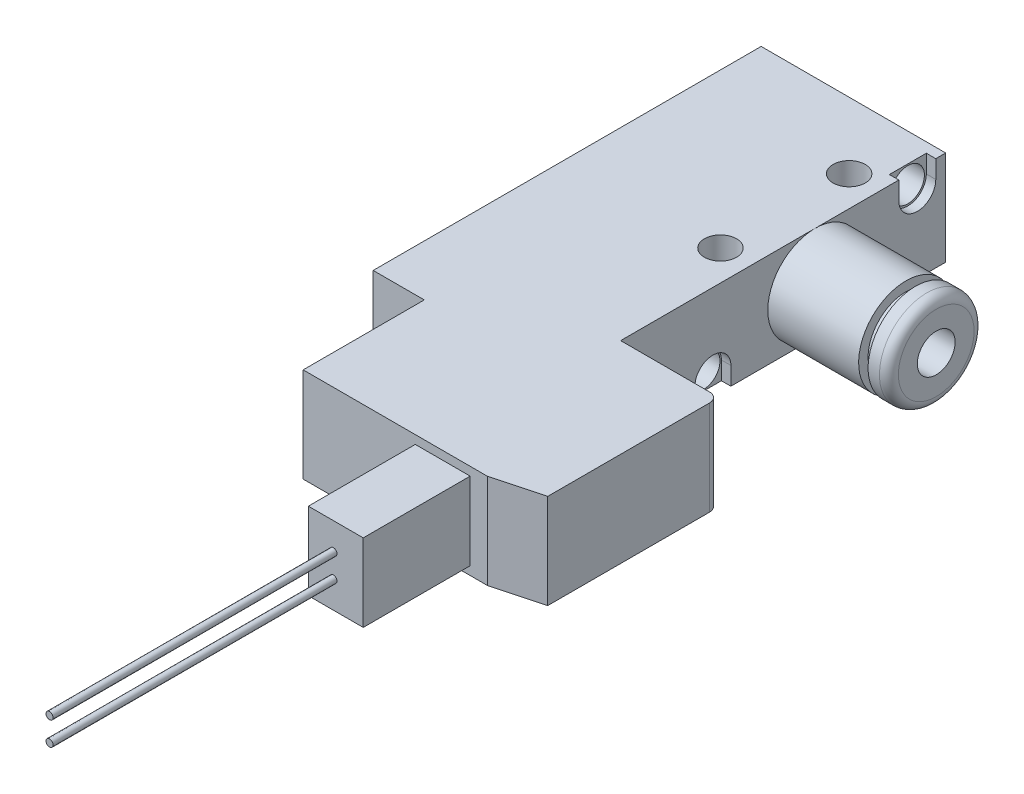
SolidWorks part; units mm, degrees
ref_plane "Front Plane" through (0, 0, 0) normal (0, 0, 1) x (1, 0, 0)
ref_plane "Top Plane" through (0, 0, 0) normal (0, 1, 0) x (1, 0, 0)
ref_plane "Right Plane" through (0, 0, 0) normal (1, 0, 0) x (0, 0, -1)
sketch "Sketch1" plane through (0, 0, 0) normal (1, 0, 0) x (0, 0, -1)
  line L1 (-26.9, 5) -> (26.9, 5)
  line L2 (-26.9, 5) -> (-26.9, -5)
  line L3 (-26.9, -5) -> (26.9, -5)
  line L4 (26.9, 5) -> (26.9, -5)
  line L5 (-26.9, 5) -> (26.9, -5) construction
  line L6 (-26.9, -5) -> (26.9, 5) construction
  point P0 (0, 0)
  dimension "D1" = 53.8
  dimension "D2" = 10
extrude "Boss-Extrude1" add sketch "Sketch1" along normal blind 29.9
sketch "Sketch2" plane through (0, -5, 0) normal (0, -1, 0) x (1, 0, 0)
  line L0 (29.9, -26.9) -> (0, -26.9) construction
  line L1 (0, 26.9) -> (0, -26.9) construction
  circle A0 centre (16.3, -19.9) radius 1.7
  circle A1 centre (16.3, -6.3) radius 1.7
  dimension "D1" = 13.6
  dimension "D3" = 3.4
  dimension "D4" = 3.4
  dimension "D2" = 7
  dimension "D5" = 16.3
extrude "Cut-Extrude1" cut sketch "Sketch2" against normal blind 29.9
sketch "Sketch3" plane through (0, 0, 26.9) normal (0, 0, 1) x (1, 0, 0)
  line L1 (0, 5) -> (0, -5) construction
  line L2 (17.25, 4.1) -> (23.05, 4.1)
  line L3 (17.25, 4.1) -> (17.25, -4.1)
  line L4 (17.25, -4.1) -> (23.05, -4.1)
  line L5 (23.05, 4.1) -> (23.05, -4.1)
  line L6 (17.25, 4.1) -> (23.05, -4.1) construction
  line L7 (17.25, -4.1) -> (23.05, 4.1) construction
  point P0 (20.15, 0)
  dimension "D1" = 17.25
  dimension "D2" = 5.8
  dimension "D3" = 8.2
sketch "Sketch5" plane through (0, -5, 0) normal (0, -1, 0) x (1, 0, 0)
  line L0 (29.9, -26.9) -> (0, -26.9) construction
  line L1 (0, 26.9) -> (5.4, 26.9)
  line L2 (0, 26.9) -> (0, 14.1)
  line L3 (0, 14.1) -> (5.4, 14.1)
  line L4 (5.4, 26.9) -> (5.4, 14.1)
  dimension "D1" = 41
  dimension "D2" = 5.4
extrude "Cut-Extrude3" cut sketch "Sketch5" against normal blind 30
hole_wizard "M5 Tapped Hole1" positions "3DSketch1" profile "Sketch6" tap size "M5" standard "Gb"
sketch3d "3DSketch1"
  line L0 (0, 5, -26.9) -> (0, 5, 14.1) construction
  line L1 (0, -5, -26.9) -> (0, 5, -26.9) construction
  point P0 (0, 0, -17.9)
  point P2 (0, 0, -7.2)
  point P4 (0, 0, 5.1)
  dimension "D1" = 5
  dimension "D2" = 5
  dimension "D3" = 5
  dimension "D4" = 9
  dimension "D5" = 10.7
  dimension "D6" = 32
sketch "Sketch6" plane through (0, 0, -17.9) normal (0, 1, 0) x (0, 0, 1)
  line L0 (0, 0) -> (0, 13.6618)
  line L1 (0, 13.6618) -> (2.1, 12.4)
  line L2 (2.1, 12.4) -> (2.1, 0)
  line L5 (2.1, 0) -> (0, 0)
  line L10 (0, 13.6618) -> (-2.1, 12.4) construction
  line L11 (0, -6.35) -> (0, 107.95) construction
  dimension "螺纹孔钻头直径" = 4.2
  dimension "螺纹孔钻头深度" = 12.4
  dimension "导头角度" = 118
cosmetic thread "Hole Thread1" parameters "D1"=10, "D2"=5
cosmetic thread "Hole Thread2" parameters "D1"=10, "D2"=5
cosmetic thread "Hole Thread3" parameters "D1"=10, "D2"=5
extrude "Boss-Extrude4" add sketch "Sketch3" along normal blind 11.3
sketch "Sketch7" plane through (0, 0, 38.2) normal (0, 0, 1) x (1, 0, 0)
  line L0 (17.25, 4.1) -> (17.25, -4.1) construction
  circle A0 centre (19.9, 1.25) radius 0.375
  circle A1 centre (19.9, -1.25) radius 0.375
  dimension "D1" = 0.75
  dimension "D2" = 0.75
  dimension "D3" = 2.5
  dimension "D4" = 2.65
  dimension "D5" = 1.25
extrude "Boss-Extrude5" add sketch "Sketch7" along normal blind 30
sketch "Sketch8" plane through (0, -5, 0) normal (0, -1, 0) x (1, 0, 0)
  line L1 (29.9, -26.9) -> (19.5, -26.9)
  line L2 (29.9, -26.9) -> (29.9, 7.45)
  line L3 (29.9, 7.45) -> (19.5, 7.45)
  line L4 (19.5, -26.9) -> (19.5, 7.45)
  dimension "D1" = 10.4
  dimension "D2" = 34.35
extrude "Cut-Extrude4" cut sketch "Sketch8" against normal blind 30
sketch "Sketch9" plane through (19.5, 0, 0) normal (1, 0, 0) x (0, 0, -1)
  line L0 (26.9, 5) -> (26.9, -5) construction
  circle A0 centre (13.1, 0) radius 5
  circle A1 centre (13.1, 0) radius 2
  dimension "D2" = 10
  dimension "D3" = 4
  dimension "D1" = 13.8
extrude "Boss-Extrude6" add sketch "Sketch9" along normal blind 12.8
fillet "Fillet1" radius 1 1 edges at (32.3, 0, -18.1)
fillet "Fillet2" radius 1 1 edges at (29.9, 0, 7.45)
chamfer "Chamfer2" distance 5 angle 15 1 edges at (29.9, 0, 26.9)
sketch "Sketch11" plane through (0, 0, 0) normal (0, 1, 0) x (1, 0, 0)
  line L0 (19.5, 8.1) -> (31.3, 8.1) construction
  line L1 (30.1, 8.1) -> (29.1, 8.1)
  line L2 (30.1, 8.1) -> (30.1, 9.1)
  line L3 (30.1, 9.1) -> (29.1, 9.1)
  line L4 (29.1, 8.1) -> (29.1, 9.1)
  line L5 (32.3, 9.1) -> (32.3, 17.1) construction
  dimension "D1" = 3.2
  dimension "D2" = 1
  dimension "D3" = 1
revolve "Cut-Revolve1" cut sketch "Sketch11" angle 360 about axis through (32.3, 0, -13.1) along (-1, 0, 0)
sketch "Sketch12" plane through (19.5, 0, 0) normal (1, 0, 0) x (0, 0, -1)
  line L0 (26.9, 5) -> (26.9, -5) construction
  circle A0 centre (23.9, 3.1) radius 1.75
  circle A1 centre (2.3, -3.1) radius 1.75
  dimension "D1" = 3.5
  dimension "D6" = 3.5
  dimension "D2" = 3.1
  dimension "D3" = 3
  dimension "D4" = 24.6
  dimension "D5" = 3.1
extrude "Cut-Extrude5" cut sketch "Sketch12" against normal blind 10
sketch "Sketch13" plane through (19.5, 0, 0) normal (1, 0, 0) x (0, 0, -1)
  line L0 (4.2, -3.1) -> (4.2, -5)
  line L1 (-7.45, -5) -> (13.1, -5) construction
  line L2 (0.4, -3.1) -> (0.4, -5)
  line L3 (25.8527, 3.1) -> (25.8527, 5)
  line L4 (13.1, 5) -> (26.9, 5) construction
  line L5 (21.9473, 3.1) -> (21.9473, 5)
  line L6 (21.9473, 5) -> (25.8527, 5)
  line L7 (0.4, -5) -> (4.2, -5)
  arc A0 (4.2, -3.1) -> (0.4, -3.1) centre (2.3, -3.1) ccw
  arc A1 (21.9473, 3.1) -> (25.8527, 3.1) centre (23.9, 3.1) ccw
extrude "Cut-Extrude6" cut sketch "Sketch13" against normal blind 1
